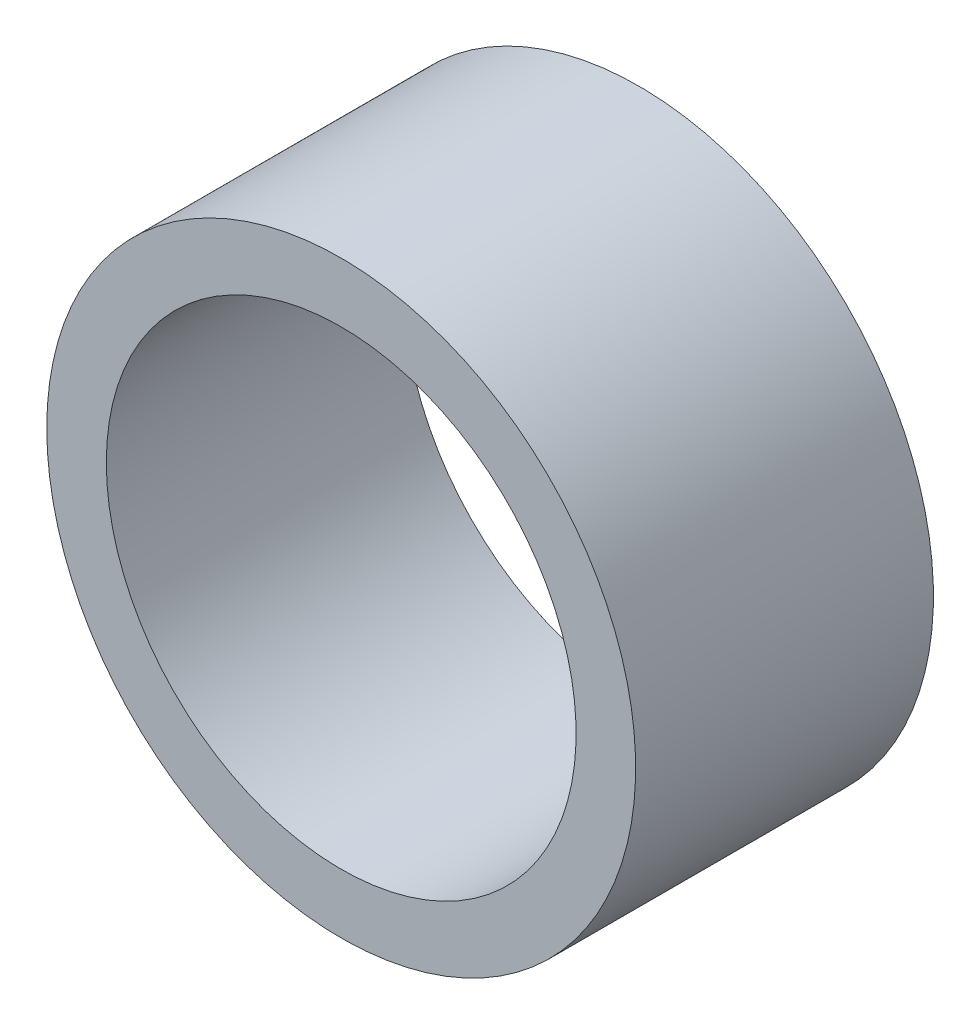
from build123d import *

# Parameters (mm, degrees)
SKETCH1_R           = 44.5
SKETCH1_R_2         = 35.5
BOSS_EXTRUDE1_DEPTH = 45


with BuildPart() as part:
    # Sketch1 → Boss-Extrude1 (new body)
    with BuildSketch(Plane.XY):
        with Locations(Location((0, 0, 0), (0, 0, 180))):
            Circle(SKETCH1_R)
        with Locations(Location((0, 0, 0), (0, 0, 180))):
            Circle(SKETCH1_R_2, mode=Mode.SUBTRACT)
    extrude(amount=BOSS_EXTRUDE1_DEPTH)


solid = part.part
